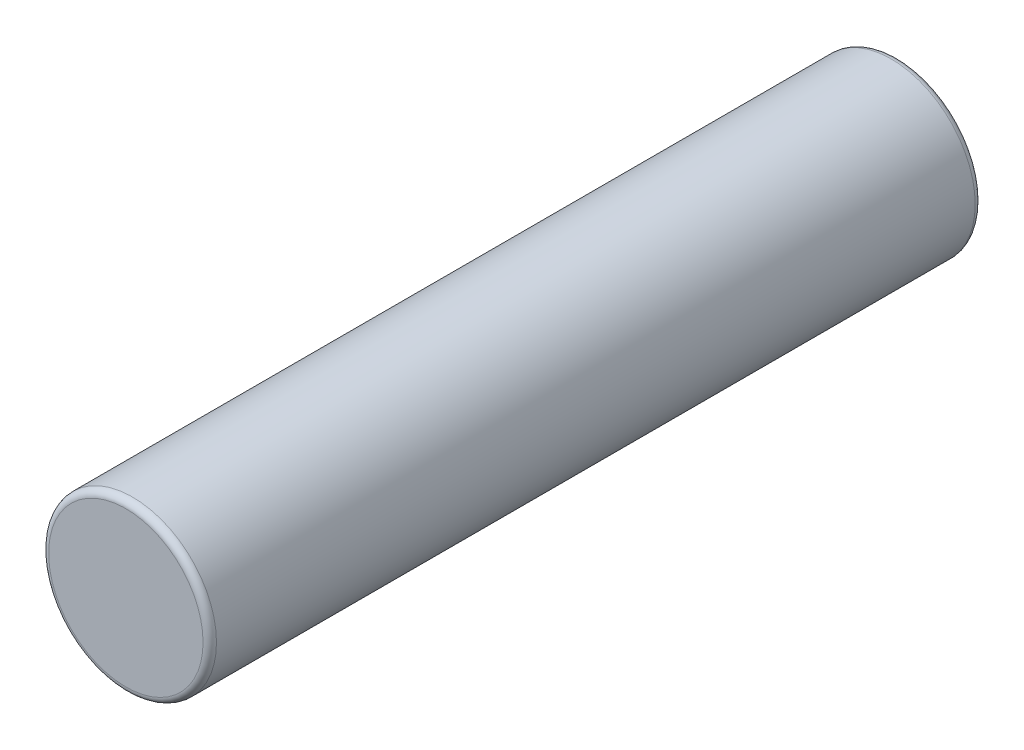
from build123d import *

# Parameters (mm, degrees)
SKETCH_1_R      = 2.5
EXTRUDE_1_DEPTH = 23
FILLET_1_R      = 0.2


with BuildPart() as part:
    # 草图1 → 凸台-拉伸1 (new body)
    with BuildSketch(Plane.XY):
        Circle(SKETCH_1_R)
    extrude(amount=EXTRUDE_1_DEPTH)

    # 圆角1
    fillet_1_edges = [part.edges().sort_by_distance(p)[0] for p in [
        (-2.5, 0, 0),
        (-2.5, 0, 23),
    ]]
    fillet(fillet_1_edges, radius=FILLET_1_R)


solid = part.part
